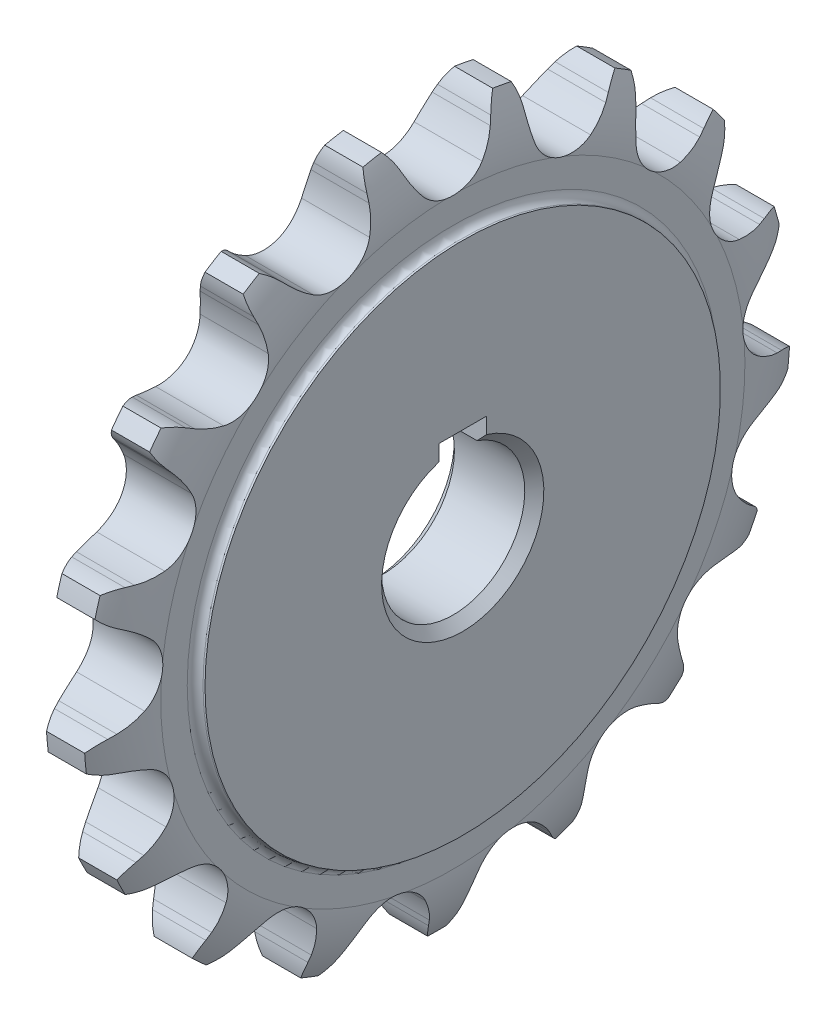
SolidWorks part; units mm, degrees
ref_plane "前视基准面" through (0, 0, 0) normal (0, 0, 1) x (1, 0, 0)
ref_plane "上视基准面" through (0, 0, 0) normal (0, 1, 0) x (1, 0, 0)
ref_plane "右视基准面" through (0, 0, 0) normal (1, 0, 0) x (0, 0, -1)
sketch "草图1" plane through (0, 0, 0) normal (0, 0, 1) x (1, 0, 0)
  line L0 (-6.35, 0) -> (6.35, 0) construction
  line L1 (-4.6852, 7.5) -> (-4.6852, 27)
  line L2 (-4.6852, 27) -> (-4.4782, 27)
  line L3 (-3.6502, 27.8279) -> (-3.6502, 30.5979)
  line L4 (-1.9992, 37) -> (1.9992, 37)
  line L5 (3.6502, 30.5979) -> (3.6502, 27.8279)
  line L6 (4.4782, 27) -> (4.6852, 27)
  line L7 (4.6852, 27) -> (4.6852, 7.5)
  line L8 (4.6852, 7.5) -> (-4.6852, 7.5)
  line L9 (0, 0) -> (0, 37) construction
  line L10 (-3.0626, 34.5579) -> (3.0626, 34.5579) construction
  line L11 (-3.0626, -34.5579) -> (3.0626, -34.5579) construction
  line L12 (6.35, 0) -> (23.35, 0) construction
  line L13 (-3.6502, 30.5979) -> (3.7984, 30.5979) construction
  line L14 (-3.6502, -30.5979) -> (3.7984, -30.5979) construction
  line L15 (23.35, 0) -> (31.27, 0) construction
  line L16 (31.27, 0) -> (43.34, 0) construction
  line L17 (43.34, 0) -> (51.19, 0) construction
  line L18 (51.19, 0) -> (65.57, 0) construction
  arc A0 (-1.9992, 37) -> (-3.6502, 30.5979) centre (9.049, 30.7369) ccw
  arc A1 (1.9992, 37) -> (3.6502, 30.5979) centre (-9.049, 30.7369) cw
  arc A2 (3.6502, 27.8279) -> (4.4782, 27) centre (4.4782, 27.8279) ccw
  arc A3 (-4.4782, 27) -> (-3.6502, 27.8279) centre (-4.4782, 27.8279) ccw
  point P30 (3.6502, 27)
  point P33 (-3.6502, 27)
  dimension "D1" = 3.5979
  dimension "rx" = 12.7
  dimension "D3" = 0.8279
  dimension "d" = 69.1158
  dimension "p" = 12.7
  dimension "z" = 17
  dimension "da" = 74
  dimension "df" = 61.1958
  dimension "dr" = 7.92
  dimension "dk" = 15
  dimension "dg" = 54
  dimension "h" = 12.07
  dimension "bf1" = 7.3005
  dimension "b1" = 7.85
  dimension "ba" = 1.651
  dimension "D2" = 1.0349
  dimension "pt" = 14.38
revolve "旋转1" add sketch "草图1" angle 360 about L0
sketch "草图2" plane through (0, 0, 0) normal (1, 0, 0) x (0, 0, -1)
  line L0 (0, 0) -> (0, 37) construction
  line L1 (0, 0) -> (-6.7987, 36.37) construction
  line L2 (0, 0) -> (-13.3659, 34.5015) construction
  line L3 (3.1525, 32.0477) -> (1.2637, 33.5517) construction
  line L4 (4.526, 34.3177) -> (-4.9566, 38.5047) construction
  line L5 (0, 0) -> (6.7987, 36.37) construction
  line L6 (4.526, 34.3177) -> (4.8285, 35.0028)
  line L7 (-4.526, 34.3177) -> (-4.8285, 35.0028)
  circle A0 centre (0, 0) radius 37 construction
  arc A1 (3.1525, 32.0477) -> (-3.1525, 32.0477) centre (0, 34.5579) cw
  arc A2 (3.1525, 32.0477) -> (4.526, 34.3177) centre (-4.9566, 38.5047) ccw
  arc A3 (5.8231, 36.5389) -> (4.8285, 35.0028) centre (10.1207, 32.666) ccw
  arc A4 (-3.1525, 32.0477) -> (-4.526, 34.3177) centre (4.9566, 38.5047) cw
  arc A5 (-5.8231, 36.5389) -> (-4.8285, 35.0028) centre (-10.1207, 32.666) cw
  arc A7 (5.8231, 36.5389) -> (-5.8231, 36.5389) centre (0, 0) ccw
  dimension "r1" = 4.0298
  dimension "r3" = 5.7852
  dimension "D1" = 21.176
  dimension "D2" = 10.588
  dimension "α/2" = 51.471
  dimension "M" = 4.9566
  dimension "T" = 3.9468
  dimension "β" = 14.706
  dimension "γ/2" = 13.235
  dimension "bc" = 0.7488
extrude "切除-拉伸1" cut sketch "草图2" against normal mid plane 9.3703
pattern_circular "阵列(圆周)1" count 17 over 360 about axis through (0, 0, 0) along (1, 0, 0) of "切除-拉伸1"
sketch "草图3" plane through (0, 0, 0) normal (0, 0, 1) x (1, 0, 0)
  line L0 (4.6852, 7.5) -> (10.3148, 7.5)
  line L3 (10.3148, 7.5) -> (10.3148, 15.4912)
  line L4 (10.3148, 15.4912) -> (4.6852, 15.4912)
  line L5 (4.6852, 15.4912) -> (4.6852, 7.5)
  line L6 (0, 0) -> (4.8, 0) construction
  line L8 (-4.6852, 27) -> (-4.6852, -27) construction
  dimension "h" = 7.9912
  dimension "K" = 4.8
  dimension "L" = 15
revolve "旋转2" [suppressed] add sketch "草图3" angle 360 about L6
sketch "草图4" plane through (-4.6852, 0, 0) normal (-1, 0, 0) x (0, 0, 1)
  line L1 (-2.5, 7.0711) -> (2.5, 7.0711)
  line L2 (-2.5, 7.0711) -> (-2.5, 9.8)
  line L3 (-2.5, 9.8) -> (2.5, 9.8)
  line L4 (2.5, 7.0711) -> (2.5, 9.8)
  circle A0 centre (0, 0) radius 7.5 construction
  point P6 (0.2, 9.8)
  dimension "D1" = 9.8
  dimension "键槽宽度" = 5
  dimension "t1" = 2.3
extrude "切除-拉伸2" cut sketch "草图4" against normal through all
chamfer "倒角1" distance 1 angle 45 1 edges at (-4.6852, -7.5, 0)
chamfer "倒角2" distance 1 angle 45 1 edges at (4.6852, -7.5, 0)
chamfer "倒角3" [suppressed] distance 1 angle 45
